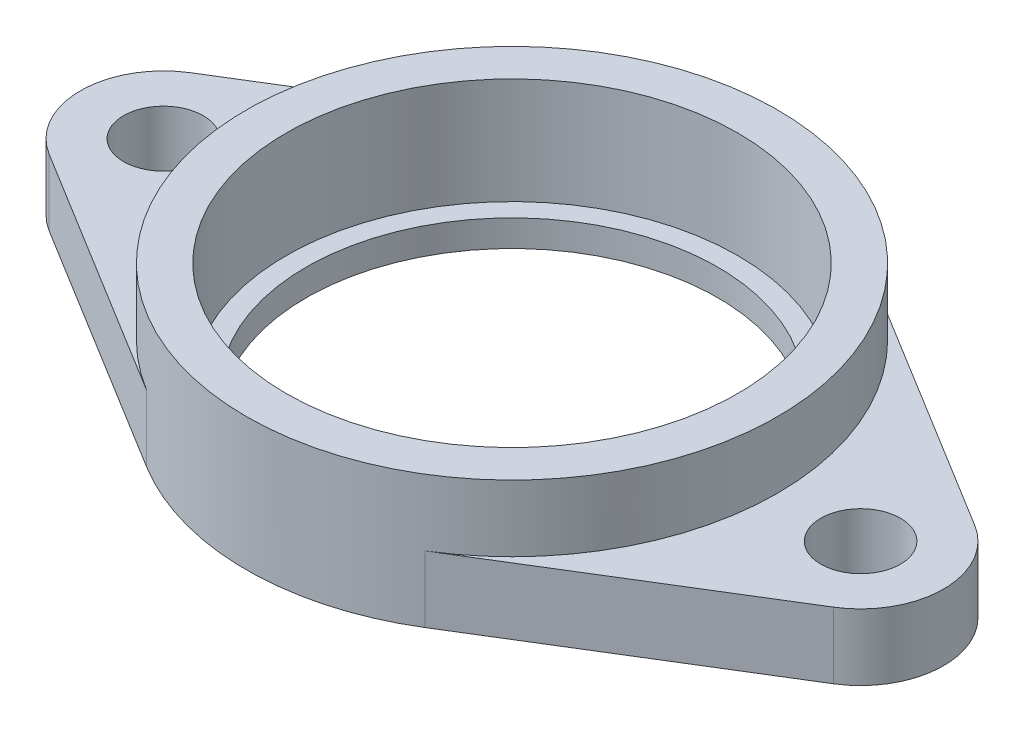
SolidWorks part; units mm, degrees
ref_plane "前视基准面" through (0, 0, 0) normal (0, 0, 1) x (1, 0, 0)
ref_plane "上视基准面" through (0, 0, 0) normal (0, 1, 0) x (1, 0, 0)
ref_plane "右视基准面" through (0, 0, 0) normal (1, 0, 0) x (0, 0, -1)
sketch "草图1" plane through (0, 0, 0) normal (0, 1, 0) x (1, 0, 0)
  line L0 (-59.0476, 10.6479) -> (-20.9524, 34.0734)
  line L1 (20.9524, 34.0734) -> (59.0476, 10.6479)
  line L2 (59.0476, -10.6479) -> (20.9524, -34.0734)
  line L3 (-20.9524, -34.0734) -> (-59.0476, -10.6479)
  arc A0 (-20.9524, -34.0734) -> (20.9524, -34.0734) centre (0, 0) ccw
  arc A1 (-59.0476, 10.6479) -> (-59.0476, -10.6479) centre (-52.5, 0) ccw
  circle A2 centre (52.5, 0) radius 6
  arc A3 (59.0476, -10.6479) -> (59.0476, 10.6479) centre (52.5, 0) ccw
  circle A4 centre (-52.5, 0) radius 6
  arc A5 (20.9524, 34.0734) -> (-20.9524, 34.0734) centre (0, 0) ccw
extrude "凸台-拉伸1" add sketch "草图1" along normal blind 10
sketch "草图2" plane through (0, 10, 0) normal (0, 1, 0) x (1, 0, 0)
  circle A0 centre (0, 0) radius 40
extrude "凸台-拉伸2" add sketch "草图2" along normal blind 10
sketch "草图3" plane through (0, 20, 0) normal (0, 1, 0) x (1, 0, 0)
  circle A0 centre (0, 0) radius 34
extrude "切除-拉伸1" cut sketch "草图3" against normal blind 16
sketch "草图4" plane through (0, 4, 0) normal (0, 1, 0) x (1, 0, 0)
  circle A0 centre (0, 0) radius 31
extrude "切除-拉伸2" cut sketch "草图4" against normal blind 16
